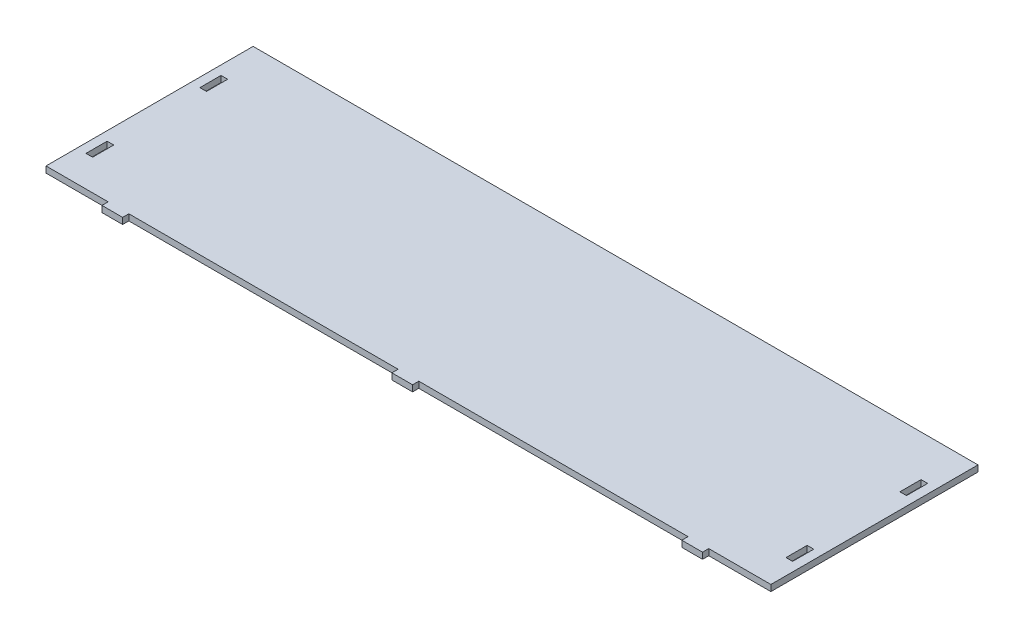
from build123d import *

# Parameters (mm, degrees)
SKETCH1_W           = 350
SKETCH1_H           = 100
BOSS_EXTRUDE1_DEPTH = 3
SKETCH2_W           = 3.2
SKETCH2_H           = 10.2
CUT_EXTRUDE1_DEPTH  = 183.027470454
SKETCH3_W           = 10
SKETCH3_H           = 3
BOSS_EXTRUDE2_DEPTH = 3


with BuildPart() as part:
    # Sketch1 → Boss-Extrude1 (new body)
    with BuildSketch(Plane(origin=(0, 0, 0), x_dir=(1, 0, 0), z_dir=(0, 1, 0))):
        Rectangle(SKETCH1_W, SKETCH1_H)
    extrude(amount=BOSS_EXTRUDE1_DEPTH)

    # Sketch2 → Cut-Extrude1 (cut, through all)
    with BuildSketch(Plane(origin=(0, 3, 0), x_dir=(1, 0, 0), z_dir=(0, 1, 0))):
        with Locations((-169, 25)):
            Rectangle(SKETCH2_W, SKETCH2_H)
        with Locations((-169, -30)):
            Rectangle(SKETCH2_W, SKETCH2_H)
        with Locations((169, -30)):
            Rectangle(SKETCH2_W, SKETCH2_H)
        with Locations((169, 25)):
            Rectangle(SKETCH2_W, SKETCH2_H)
    extrude(amount=-CUT_EXTRUDE1_DEPTH, mode=Mode.SUBTRACT)

    # Sketch3 → Boss-Extrude2 (add)
    with BuildSketch(Plane(origin=(0, 3, 0), x_dir=(1, 0, 0), z_dir=(0, 1, 0))):
        with Locations((-140, -51.5)):
            Rectangle(SKETCH3_W, SKETCH3_H)
        with Locations((0, -51.5)):
            Rectangle(SKETCH3_W, SKETCH3_H)
        with Locations((140, -51.5)):
            Rectangle(SKETCH3_W, SKETCH3_H)
    extrude(amount=-BOSS_EXTRUDE2_DEPTH)


solid = part.part
